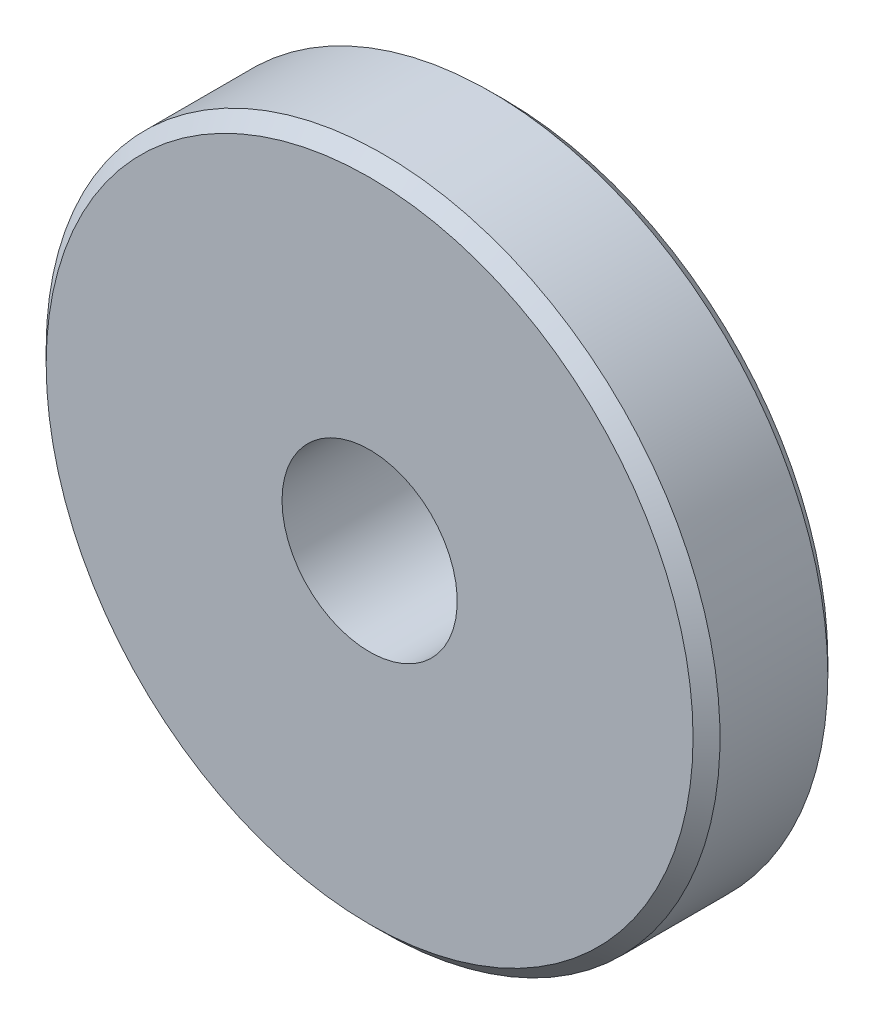
SolidWorks part; units mm, degrees
ref_plane "前视基准面" through (0, 0, 0) normal (0, 0, 1) x (1, 0, 0)
ref_plane "上视基准面" through (0, 0, 0) normal (0, 1, 0) x (1, 0, 0)
ref_plane "右视基准面" through (0, 0, 0) normal (1, 0, 0) x (0, 0, -1)
sketch "草图1" plane through (0, 0, 0) normal (0, 0, 1) x (1, 0, 0)
  circle A0 centre (0, 0) radius 12.5
  circle A1 centre (0, 0) radius 3.25
  dimension "D1" = 25
  dimension "D2" = 6.5
extrude "凸台-拉伸1" add sketch "草图1" along normal mid plane 5
chamfer "倒角1" distance 0.5 angle 45 2 edges at (12.5, 0, 2.5) (12.5, 0, -2.5)
